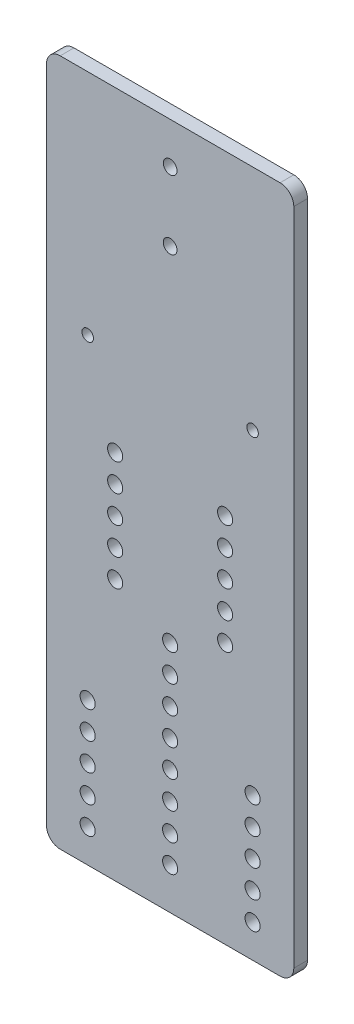
SolidWorks part; units mm, degrees
ref_plane "前视基准面" through (0, 0, 0) normal (0, 0, 1) x (1, 0, 0)
ref_plane "上视基准面" through (0, 0, 0) normal (0, 1, 0) x (1, 0, 0)
ref_plane "右视基准面" through (0, 0, 0) normal (1, 0, 0) x (0, 0, -1)
sketch "草图1" plane through (0, 0, 0) normal (0, 0, 1) x (1, 0, 0)
  line L1 (-45, 125) -> (45, 125)
  line L2 (-45, 125) -> (-45, -125)
  line L3 (-45, -125) -> (45, -125)
  line L4 (45, 125) -> (45, -125)
  line L5 (-45, 125) -> (45, -125) construction
  line L6 (-45, -125) -> (45, 125) construction
  point P0 (0, 0)
  dimension "D1" = 90
  dimension "D2" = 250
extrude "凸台-拉伸1" add sketch "草图1" along normal blind 5
sketch "草图2" plane through (0, 0, 5) normal (0, 0, 1) x (1, 0, 0)
  line L0 (0, -125) -> (0, 110) construction
  line L1 (-45, -125) -> (45, -125) construction
  line L2 (45, 125) -> (-45, 125) construction
  line L3 (-30, 42) -> (0, 42) construction
  line L4 (0, 42) -> (30, 42) construction
  circle A0 centre (0, 110) radius 2.5
  circle A1 centre (0, 85) radius 2.5
  circle A2 centre (-30, 42) radius 2.1
  circle A3 centre (30, 42) radius 2.1
  dimension "D1" = 5
  dimension "D2" = 15
  dimension "D3" = 25
  dimension "D4" = 4.2
  dimension "D6" = 60
  dimension "D5" = 43
extrude "切除-拉伸1" cut sketch "草图2" against normal blind 5
sketch "草图3" plane through (0, 0, 5) normal (0, 0, 1) x (1, 0, 0)
  line L0 (0, 0) -> (0, -30) construction
  line L1 (0, -30) -> (-20, -30) construction
  line L2 (0, -30) -> (20, -30) construction
  line L3 (0, -30) -> (0, -80) construction
  circle A0 centre (-20, -30) radius 2.75
  circle A1 centre (20, -30) radius 2.75
  circle A2 centre (-30, 42) radius 2.1 construction
  circle A3 centre (0, -80) radius 2.75
  circle A4 centre (0, -70) radius 2.75
  circle A5 centre (0, -60) radius 2.75
  circle A6 centre (0, -50) radius 2.75
  circle A7 centre (0, -40) radius 2.75
  circle A66 centre (0, -90) radius 2.75
  circle A67 centre (0, -100) radius 2.75
  circle A68 centre (0, -110) radius 2.75
  circle A69 centre (-20, -20) radius 2.75
  circle A70 centre (20, -20) radius 2.75
  circle A71 centre (-20, -10) radius 2.75
  circle A72 centre (20, -10) radius 2.75
  circle A73 centre (-20, 0) radius 2.75
  circle A74 centre (20, 0) radius 2.75
  circle A75 centre (-20, 10) radius 2.75
  circle A76 centre (20, 10) radius 2.75
  dimension "D2" = 5.5
  dimension "D1" = 40
  dimension "D3" = 72
  dimension "D4" = 50
  dimension "D5" = 5
  dimension "D6" = 1
  dimension "D7" = 4
extrude "切除-拉伸2" cut sketch "草图3" against normal blind 5
sketch "草图4" plane through (0, 0, 5) normal (0, 0, 1) x (1, 0, 0)
  line L0 (0, -125) -> (0, -113) construction
  line L1 (-45, -125) -> (45, -125) construction
  line L2 (0, -113) -> (-30, -113) construction
  line L3 (0, -113) -> (30, -113) construction
  circle A0 centre (-30, -113) radius 2.75
  circle A1 centre (30, -113) radius 2.75
  circle A2 centre (0, -110) radius 2.75 construction
  circle A3 centre (-30, -103) radius 2.75
  circle A4 centre (30, -103) radius 2.75
  circle A5 centre (-30, -93) radius 2.75
  circle A6 centre (30, -93) radius 2.75
  circle A7 centre (-30, -83) radius 2.75
  circle A8 centre (30, -83) radius 2.75
  circle A9 centre (-30, -73) radius 2.75
  circle A10 centre (30, -73) radius 2.75
  dimension "D2" = 12
  dimension "D1" = 60
  dimension "D3" = 5
extrude "切除-拉伸3" cut sketch "草图4" against normal blind 5
fillet "圆角1" radius 5 4 edges at (-45, -125, 2.5) (45, -125, 2.5) (-45, 125, 2.5) (45, 125, 2.5)
